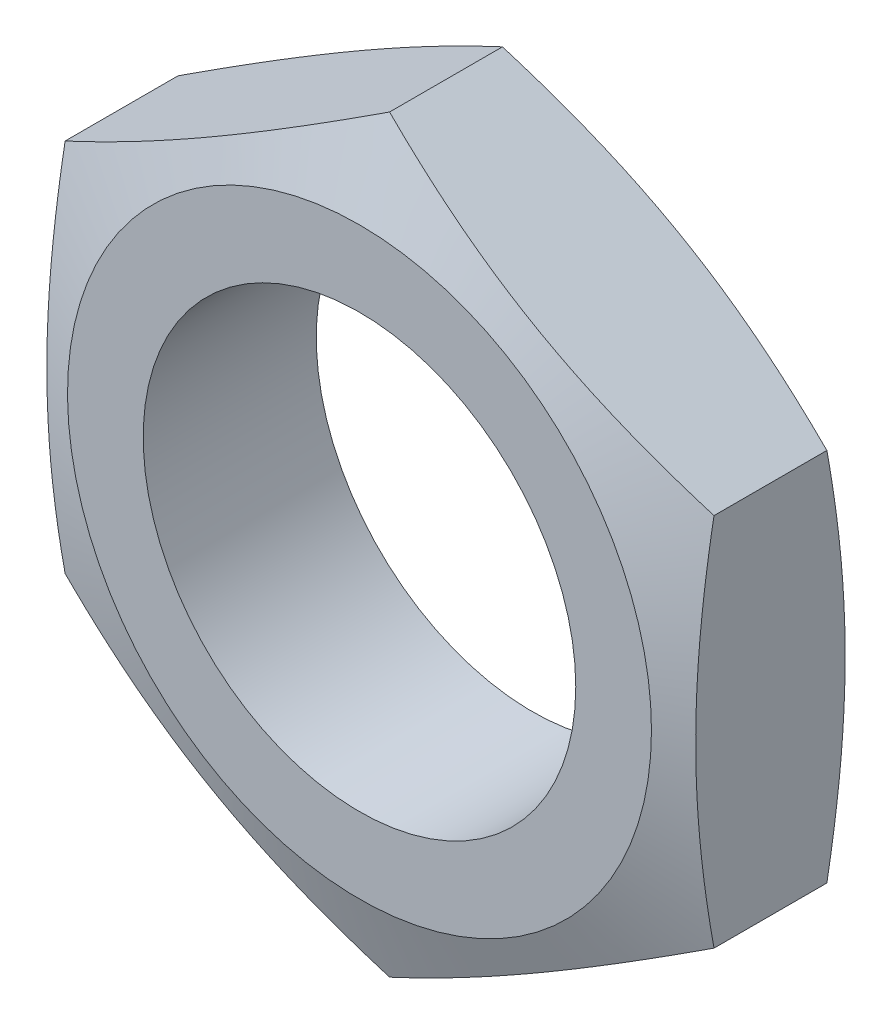
from build123d import *

# Parameters (mm, degrees)
EXTRUDE_1_DEPTH     = 8
SKETCH_5_R          = 10
CUT_EXTRUDE_1_DEPTH = 25.269322199


with BuildPart() as part:
    # 草图1 → 凸台-拉伸1 (new body)
    with BuildSketch(Plane.XY):
        Polygon((0, 17.320508076), (-15, 8.660254038), (-15, -8.660254038), (0, -17.320508076), (15, -8.660254038), (15, 8.660254038), align=None)
    extrude(amount=EXTRUDE_1_DEPTH)

    # 草图4 → 切除-旋转1 (revolve, cut)
    with BuildSketch(Plane(origin=(0, 0, 0), x_dir=(0, 0, -1), z_dir=(1, 0, 0)), mode=Mode.PRIVATE) as cut_revolve_1_sk:
        Polygon((-8, -13.5), (-6.609448781, -17.320508076), (-8, -17.320508076), align=None)
    cut_revolve_1 = revolve(cut_revolve_1_sk.sketch.rotate(Axis((0, 0, 8), (0, 0, -1)), 120.000000002), axis=Axis((0, 0, 8), (0, 0, -1)), mode=Mode.SUBTRACT)

    # 镜向1: 切除-旋转1 across plane
    add(cut_revolve_1.mirror(Plane.XY.offset(4)), mode=Mode.SUBTRACT)

    # 草图5 → 切除-拉伸1 (cut, through all)
    with BuildSketch(Plane.XY.offset(8)):
        Circle(SKETCH_5_R)
    extrude(amount=-CUT_EXTRUDE_1_DEPTH, mode=Mode.SUBTRACT)


solid = part.part
